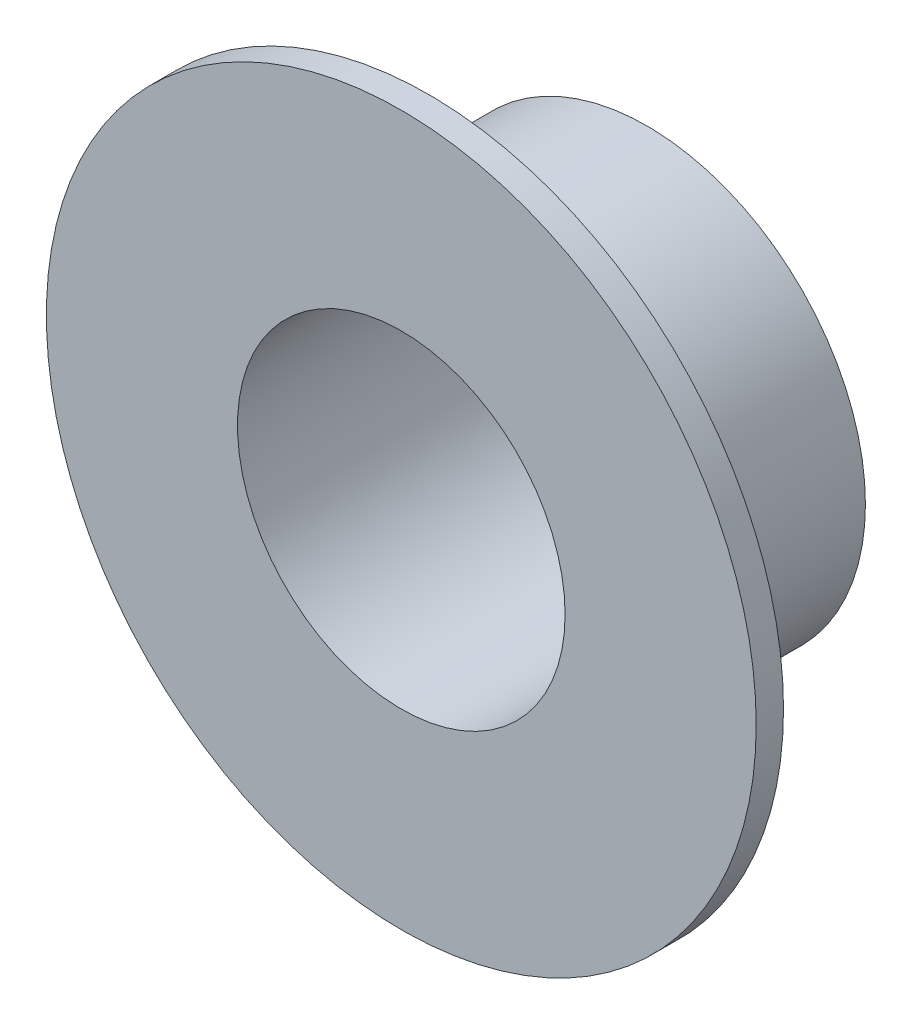
SolidWorks part; units mm, degrees
ref_plane "Front Plane" through (0, 0, 0) normal (0, 0, 1) x (1, 0, 0)
ref_plane "Top Plane" through (0, 0, 0) normal (0, 1, 0) x (1, 0, 0)
ref_plane "Right Plane" through (0, 0, 0) normal (1, 0, 0) x (0, 0, -1)
sketch "Sketch1" plane through (0, 0, 0) normal (0, 0, 1) x (1, 0, 0)
  circle A0 centre (0, 0) radius 40
  circle A1 centre (0, 0) radius 30
  dimension "D1" = 80
  dimension "D2" = 60
extrude "Boss-Extrude1" add sketch "Sketch1" along normal blind 40
sketch "Sketch2" plane through (0, 0, 40) normal (0, 0, 1) x (1, 0, 0)
  circle A0 centre (0, 0) radius 65
  circle A1 centre (0, 0) radius 30 construction
  circle A2 centre (0, 0) radius 30
  dimension "D1" = 130
extrude "Boss-Extrude2" add sketch "Sketch2" along normal blind 5
